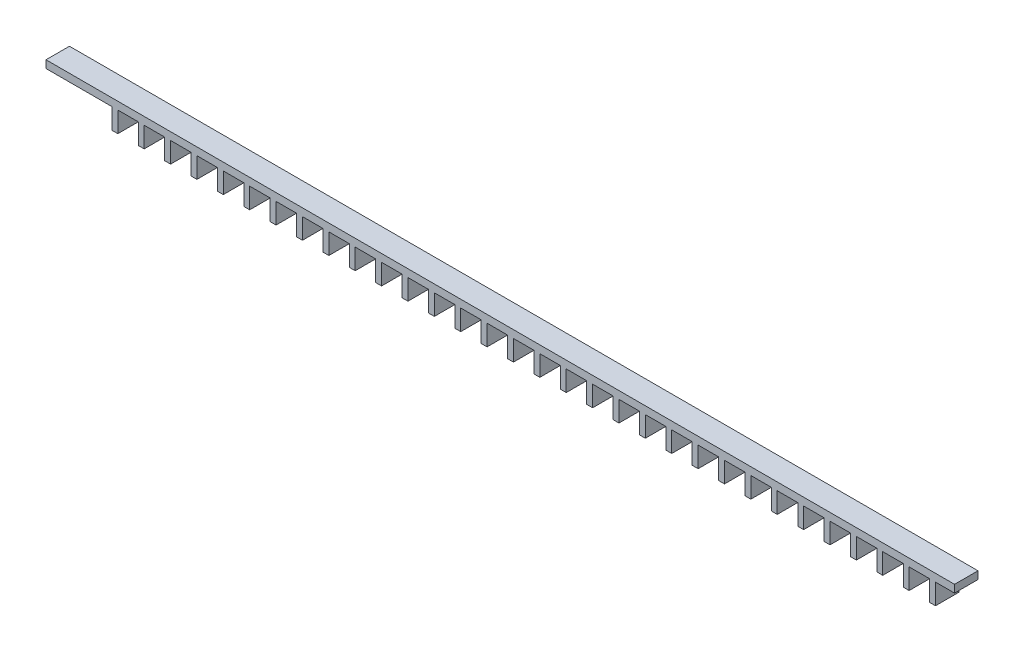
SolidWorks part; units mm, degrees
ref_plane "Front" through (0, 0, 0) normal (0, 0, 1) x (1, 0, 0)
ref_plane "Top" through (0, 0, 0) normal (0, 1, 0) x (1, 0, 0)
ref_plane "Right" through (0, 0, 0) normal (1, 0, 0) x (0, 0, -1)
sketch "草图1" plane through (0, 0, 0) normal (0, 1, 0) x (1, 0, 0)
  line L1 (-775, -20) -> (775, -20)
  line L2 (-775, -20) -> (-775, 20)
  line L3 (-775, 20) -> (775, 20)
  line L4 (775, -20) -> (775, 20)
  line L5 (-775, -20) -> (775, 20) construction
  line L6 (-775, 20) -> (775, -20) construction
  point P0 (0, 0)
  dimension "D1" = 40
  dimension "D2" = 1550
extrude "凸台-拉伸1" add sketch "草图1" along normal blind 48
sketch "草图2" plane through (0, 0, 20) normal (0, 0, 1) x (1, 0, 0)
  line L0 (-775, 0) -> (775, 0) construction
  line L1 (-770, 0) -> (-735, 0)
  line L2 (-770, 0) -> (-770, 35)
  line L3 (-770, 35) -> (-735, 35)
  line L4 (-735, 0) -> (-735, 35)
  line L5 (-725, 0) -> (-690, 0)
  line L6 (-725, 0) -> (-725, 35)
  line L7 (-725, 35) -> (-690, 35)
  line L8 (-690, 0) -> (-690, 35)
  line L9 (-680, 0) -> (-645, 0)
  line L10 (-680, 0) -> (-680, 35)
  line L11 (-680, 35) -> (-645, 35)
  line L12 (-645, 0) -> (-645, 35)
  line L13 (-635, 0) -> (-600, 0)
  line L14 (-635, 0) -> (-635, 35)
  line L15 (-635, 35) -> (-600, 35)
  line L16 (-600, 0) -> (-600, 35)
  line L17 (-590, 0) -> (-555, 0)
  line L18 (-590, 0) -> (-590, 35)
  line L19 (-590, 35) -> (-555, 35)
  line L20 (-555, 0) -> (-555, 35)
  line L21 (-545, 0) -> (-510, 0)
  line L22 (-545, 0) -> (-545, 35)
  line L23 (-545, 35) -> (-510, 35)
  line L24 (-510, 0) -> (-510, 35)
  line L25 (-500, 0) -> (-465, 0)
  line L26 (-500, 0) -> (-500, 35)
  line L27 (-500, 35) -> (-465, 35)
  line L28 (-465, 0) -> (-465, 35)
  line L29 (-455, 0) -> (-420, 0)
  line L30 (-455, 0) -> (-455, 35)
  line L31 (-455, 35) -> (-420, 35)
  line L32 (-420, 0) -> (-420, 35)
  line L33 (-410, 0) -> (-375, 0)
  line L34 (-410, 0) -> (-410, 35)
  line L35 (-410, 35) -> (-375, 35)
  line L36 (-375, 0) -> (-375, 35)
  line L37 (-365, 0) -> (-330, 0)
  line L38 (-365, 0) -> (-365, 35)
  line L39 (-365, 35) -> (-330, 35)
  line L40 (-330, 0) -> (-330, 35)
  line L41 (-320, 0) -> (-285, 0)
  line L42 (-320, 0) -> (-320, 35)
  line L43 (-320, 35) -> (-285, 35)
  line L44 (-285, 0) -> (-285, 35)
  line L45 (-275, 0) -> (-240, 0)
  line L46 (-275, 0) -> (-275, 35)
  line L47 (-275, 35) -> (-240, 35)
  line L48 (-240, 0) -> (-240, 35)
  line L50 (-775, 48) -> (-775, 0) construction
  line L64 (-230, 0) -> (-195, 0) [skipped]
  line L65 (-230, 35) -> (-195, 35) [skipped]
  line L66 (-195, 0) -> (-195, 35) [skipped]
  line L67 (-230, 0) -> (-230, 35) [skipped]
  dimension "D1" = 35
  dimension "D2" = 35
  dimension "D4" = 5
  dimension "D3" = 13
extrude "切除-拉伸1" cut sketch "草图2" against normal through all
sketch "草图6" plane through (0, 0, 20) normal (0, 0, 1) x (1, 0, 0)
  line L0 (-240, 0) -> (775, 0) construction
  line L1 (-230, 0) -> (-195, 0)
  line L2 (-230, 0) -> (-230, 35)
  line L3 (-230, 35) -> (-195, 35)
  line L4 (-195, 0) -> (-195, 35)
  line L5 (-95, 0) -> (-60, 0)
  line L6 (-95, 0) -> (-95, 35)
  line L7 (-95, 35) -> (-60, 35)
  line L8 (-240, 0) -> (-240, 35) construction
  line L9 (-185, 0) -> (-150, 0)
  line L10 (-185, 0) -> (-185, 35)
  line L11 (-185, 35) -> (-150, 35)
  line L12 (-150, 0) -> (-150, 35)
  line L13 (-140, 0) -> (-105, 0)
  line L14 (-140, 0) -> (-140, 35)
  line L15 (-140, 35) -> (-105, 35)
  line L16 (-105, 0) -> (-105, 35)
  line L17 (-60, 0) -> (-60, 35)
  line L18 (-50, 0) -> (-15, 0)
  line L19 (-50, 0) -> (-50, 35)
  line L20 (-50, 35) -> (-15, 35)
  line L21 (-15, 0) -> (-15, 35)
  line L22 (-5, 0) -> (30, 0)
  line L23 (-5, 0) -> (-5, 35)
  line L24 (-5, 35) -> (30, 35)
  line L25 (30, 0) -> (30, 35)
  line L26 (40, 0) -> (75, 0)
  line L27 (40, 0) -> (40, 35)
  line L28 (40, 35) -> (75, 35)
  line L29 (75, 0) -> (75, 35)
  line L30 (85, 0) -> (120, 0)
  line L31 (85, 0) -> (85, 35)
  line L32 (85, 35) -> (120, 35)
  line L33 (120, 0) -> (120, 35)
  line L34 (130, 0) -> (165, 0)
  line L35 (130, 0) -> (130, 35)
  line L36 (130, 35) -> (165, 35)
  line L37 (165, 0) -> (165, 35)
  line L38 (175, 0) -> (210, 0)
  line L39 (175, 0) -> (175, 35)
  line L40 (175, 35) -> (210, 35)
  line L41 (210, 0) -> (210, 35)
  line L42 (220, 0) -> (255, 0)
  line L43 (220, 0) -> (220, 35)
  line L44 (220, 35) -> (255, 35)
  line L45 (255, 0) -> (255, 35)
  line L46 (265, 0) -> (300, 0)
  line L47 (265, 0) -> (265, 35)
  line L48 (265, 35) -> (300, 35)
  line L49 (300, 0) -> (300, 35)
  line L50 (310, 0) -> (345, 0)
  line L51 (310, 0) -> (310, 35)
  line L52 (310, 35) -> (345, 35)
  line L53 (345, 0) -> (345, 35)
  line L54 (355, 0) -> (390, 0)
  line L55 (355, 0) -> (355, 35)
  line L56 (355, 35) -> (390, 35)
  line L57 (390, 0) -> (390, 35)
  line L58 (400, 0) -> (435, 0)
  line L59 (400, 0) -> (400, 35)
  line L60 (400, 35) -> (435, 35)
  line L61 (435, 0) -> (435, 35)
  line L62 (445, 0) -> (480, 0)
  line L63 (445, 0) -> (445, 35)
  line L64 (445, 35) -> (480, 35)
  line L65 (480, 0) -> (480, 35)
  line L66 (490, 0) -> (525, 0)
  line L67 (490, 0) -> (490, 35)
  line L68 (490, 35) -> (525, 35)
  line L69 (525, 0) -> (525, 35)
  line L70 (535, 0) -> (570, 0)
  line L71 (535, 0) -> (535, 35)
  line L72 (535, 35) -> (570, 35)
  line L73 (570, 0) -> (570, 35)
  line L74 (580, 0) -> (615, 0)
  line L75 (580, 0) -> (580, 35)
  line L76 (580, 35) -> (615, 35)
  line L77 (615, 0) -> (615, 35)
  line L78 (625, 0) -> (660, 0)
  line L79 (625, 0) -> (625, 35)
  line L80 (625, 35) -> (660, 35)
  line L81 (660, 0) -> (660, 35)
  line L82 (670, 0) -> (705, 0)
  line L83 (670, 0) -> (670, 35)
  line L84 (670, 35) -> (705, 35)
  line L85 (705, 0) -> (705, 35)
  line L86 (715, 0) -> (750, 0)
  line L87 (715, 0) -> (715, 35)
  line L88 (715, 35) -> (750, 35)
  line L89 (750, 0) -> (750, 35)
  dimension "D1" = 35
  dimension "D2" = 35
  dimension "D3" = 10
  dimension "D4" = 22
extrude "切除-拉伸5" cut sketch "草图6" against normal through all
sketch "草图7" plane through (0, 0, -20) normal (0, 0, -1) x (-1, 0, 0)
  line L0 (-775, 48) -> (-775, 0) construction
  line L1 (-775, 35) -> (-665, 35)
  line L2 (-775, 35) -> (-775, -26.4458)
  line L3 (-775, -26.4458) -> (-665, -26.4458)
  line L4 (-665, 35) -> (-665, -26.4458)
  line L5 (775, 48) -> (775, 0) construction
  line L6 (775, 35) -> (685, 35)
  line L7 (775, 35) -> (775, -49.635)
  line L8 (775, -49.635) -> (685, -49.635)
  line L9 (685, 35) -> (685, -49.635)
  dimension "D1" = 110
  dimension "D2" = 90
extrude "切除-拉伸6" cut sketch "草图7" against normal through all
sketch "草图8" plane through (-775, 0, 0) normal (-1, 0, 0) x (0, 0, 1)
  line L4 (-20, 48) -> (-20, 35)
  line L5 (-20, 35) -> (20, 35)
  line L6 (20, 35) -> (20, 48)
  line L7 (20, 48) -> (-20, 48)
  line L8 (-20, 48) -> (-20, 35)
  line L9 (-20, 35) -> (20, 35)
  line L10 (20, 35) -> (20, 48)
  line L11 (20, 48) -> (-20, 48)
  dimension "D1" = 0
extrude "凸台-拉伸2" add sketch "草图8" along normal blind 10
sketch "草图9" plane through (775, 0, 0) normal (1, 0, 0) x (0, 0, -1)
  line L4 (-20, 48) -> (-20, 35)
  line L5 (-20, 35) -> (20, 35)
  line L6 (20, 35) -> (20, 48)
  line L7 (20, 48) -> (-20, 48)
  line L8 (-20, 48) -> (-20, 35)
  line L9 (-20, 35) -> (20, 35)
  line L10 (20, 35) -> (20, 48)
  line L11 (20, 48) -> (-20, 48)
  dimension "D1" = 0
extrude "切除-拉伸7" cut sketch "草图9" against normal blind 10
sketch "草图10" plane through (665, 0, 0) normal (1, 0, 0) x (0, 0, -1)
  line L4 (-20, 0) -> (20, 0)
  line L5 (20, 0) -> (20, 35)
  line L6 (20, 35) -> (-20, 35)
  line L7 (-20, 35) -> (-20, 0)
  line L8 (-20, 0) -> (20, 0)
  line L9 (20, 0) -> (20, 35)
  line L10 (20, 35) -> (-20, 35)
  line L11 (-20, 35) -> (-20, 0)
  dimension "D1" = 0
extrude "凸台-拉伸3" add sketch "草图10" along normal blind 5
sketch "草图11" plane through (-685, 0, 0) normal (-1, 0, 0) x (0, 0, 1)
  line L4 (-20, 0) -> (20, 0)
  line L5 (20, 0) -> (20, 35)
  line L6 (20, 35) -> (-20, 35)
  line L7 (-20, 35) -> (-20, 0)
  line L8 (-20, 0) -> (20, 0)
  line L9 (20, 0) -> (20, 35)
  line L10 (20, 35) -> (-20, 35)
  line L11 (-20, 35) -> (-20, 0)
  dimension "D1" = 0
extrude "凸台-拉伸4" add sketch "草图11" along normal blind 5
other "移动面1" face at (-785, 41.5, 0) face at (765, 41.5, 0) parameters "D1"=22.5
sketch "草图12" plane through (0, 0, 20) normal (0, 0, 1) x (1, 0, 0)
  line L0 (-690, 35) -> (-807.5, 35) construction
  line L1 (-735, 35) -> (-725, 35)
  line L2 (-735, 35) -> (-735, 0)
  line L3 (-735, 0) -> (-725, 0)
  line L4 (-725, 35) -> (-725, 0)
  line L6 (-690, 0) -> (-690, 35) construction
  dimension "D1" = 10
  dimension "D2" = 35
extrude "凸台-拉伸5" add sketch "草图12" against normal up to surface (40 mm away) up to face at (-10.7031, 18.25, -20)
other "移动面2" face at (-807.5, 41.5, 0) face at (742.5, 41.5, 0) parameters "D1"=40
